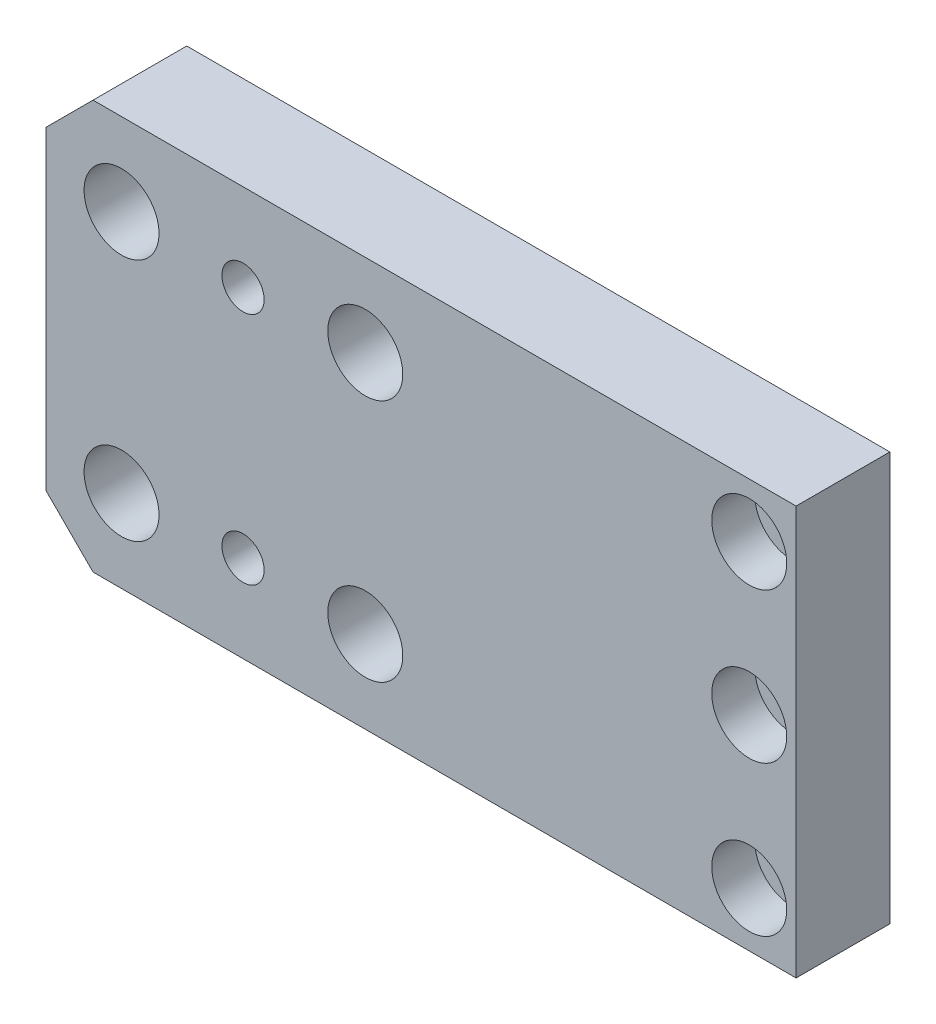
SolidWorks part; units mm, degrees
ref_plane "前视基准面" through (0, 0, 0) normal (0, 0, 1) x (1, 0, 0)
ref_plane "上视基准面" through (0, 0, 0) normal (0, 1, 0) x (1, 0, 0)
ref_plane "右视基准面" through (0, 0, 0) normal (1, 0, 0) x (0, 0, -1)
sketch "草图1" plane through (0, 0, 0) normal (0, 1, 0) x (1, 0, 0)
  line L1 (0, 0) -> (80, 0)
  line L2 (0, 0) -> (0, 10)
  line L3 (0, 10) -> (80, 10)
  line L4 (80, 0) -> (80, 10)
  dimension "D1" = 10
  dimension "D2" = 80
extrude "凸台-拉伸1" add sketch "草图1" along normal blind 43.6
chamfer "倒角1" distance 5 angle 45 2 edges at (0, 0, -5) (0, 43.6, -5)
sketch "草图6" plane through (0, 0, -10) normal (0, 0, -1) x (-1, 0, 0)
  point P0 (-34.0428, 34.8)
  point P3 (-8.0428, 34.8)
  point P6 (-8.0428, 8.8)
  point P9 (-34.0428, 8.8)
hole_wizard "Ø8.0 (8) 直径孔1" positions "草图6" profile "草图5" hole size "Ø8.0" standard "GB" end condition through all
sketch "草图5" plane through (34.0428, 34.8, -10) normal (1, 0, 0) x (0, 1, 0)
  line L0 (0, 0) -> (0, 10)
  line L1 (0, 10) -> (4, 10)
  line L2 (4, 10) -> (4, 0)
  line L5 (4, 0) -> (0, 0)
  line L11 (0, -6.35) -> (0, 107.95) construction
  dimension "通孔孔直径" = 8
  dimension "通孔孔深度" = 10
sketch "草图9" plane through (0, 0, -10) normal (0, 0, -1) x (-1, 0, 0)
  line L1 (0, 21.8) -> (-46.938, 21.8) construction
  line L2 (0, 38.6) -> (0, 5) construction
  point P0 (-21, 34.3)
  point P2 (-21, 9.3)
  dimension "D1" = 21
  dimension "D2" = 25
hole_wizard "M4 六角圆柱头螺钉的柱形沉头孔1" positions "草图9" profile "草图8" counterbore size "M4" standard "GB" end condition through all
sketch "草图8" plane through (21, 34.3, -10) normal (1, 0, 0) x (0, 1, 0)
  line L0 (0, 0) -> (0, 10)
  line L1 (0, 10) -> (2.25, 10)
  line L3 (2.25, 10) -> (2.25, 4.6)
  line L4 (2.25, 4.6) -> (4, 4.6)
  line L5 (4, 4.6) -> (4, 0)
  line L7 (4, 0) -> (0, 0)
  line L11 (0, -6.35) -> (0, 107.95) construction
  dimension "通孔孔直径" = 4.5
  dimension "通孔孔深度" = 10
  dimension "柱形沉头孔直径" = 8
  dimension "柱形沉头孔深度" = 4.6
sketch "草图12" plane through (0, 0, 0) normal (0, 0, 1) x (1, 0, 0)
  line L0 (0, 21.8) -> (97.8561, 21.8) construction
  line L1 (0, 38.6) -> (0, 5) construction
  line L3 (80, 43.6) -> (80, 0) construction
  point P0 (75, 37.8)
  point P2 (75, 5.8)
  point P4 (75, 21.8)
  dimension "D1" = 32
  dimension "D2" = 5
hole_wizard "M4 六角圆柱头螺钉的柱形沉头孔2" positions "草图12" profile "草图11" counterbore size "M4" standard "GB" end condition through all
sketch "草图11" plane through (75, 37.8, 0) normal (1, 0, 0) x (0, -1, 0)
  line L0 (0, 0) -> (0, 10)
  line L1 (0, 10) -> (2.25, 10)
  line L3 (2.25, 10) -> (2.25, 4.6)
  line L4 (2.25, 4.6) -> (4, 4.6)
  line L5 (4, 4.6) -> (4, 0)
  line L7 (4, 0) -> (0, 0)
  line L11 (0, -6.35) -> (0, 107.95) construction
  dimension "通孔孔直径" = 4.5
  dimension "通孔孔深度" = 10
  dimension "柱形沉头孔直径" = 8
  dimension "柱形沉头孔深度" = 4.6
